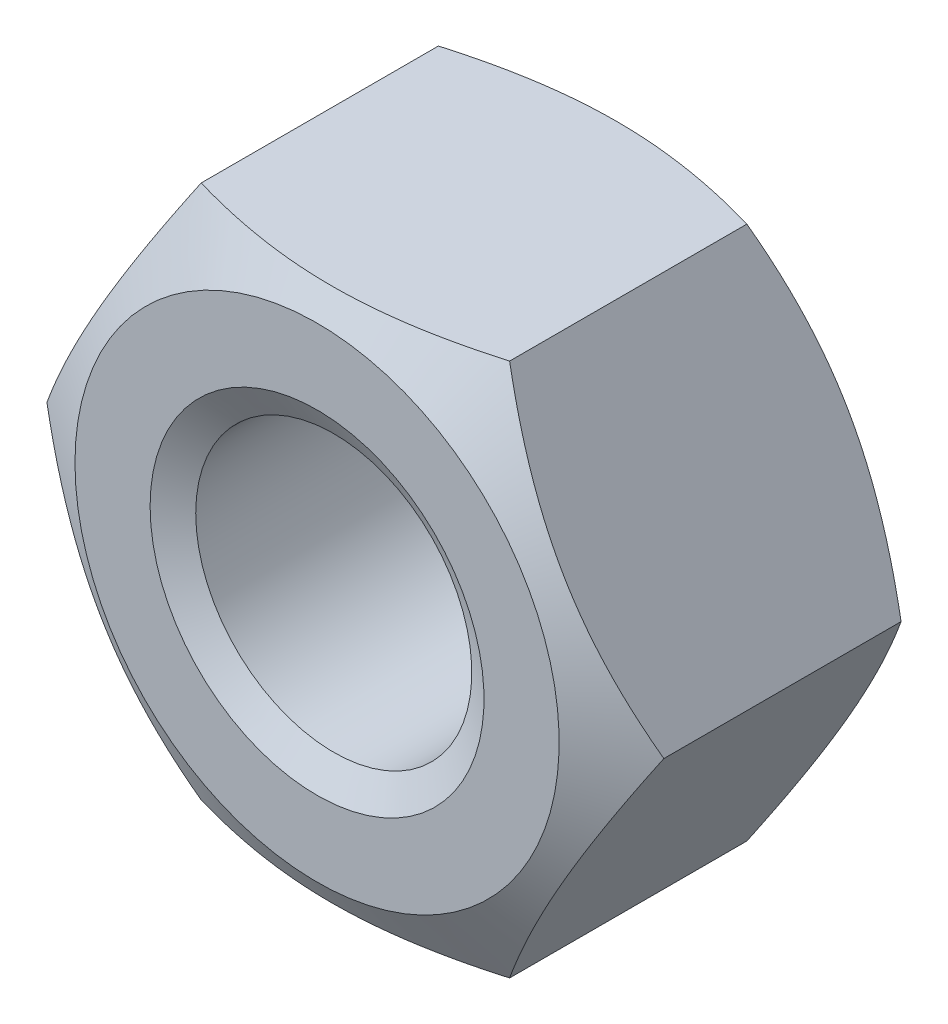
SolidWorks part; units mm, degrees
ref_plane "Front" through (0, 0, 0) normal (0, 0, 1) x (1, 0, 0)
ref_plane "Top" through (0, 0, 0) normal (0, 1, 0) x (1, 0, 0)
ref_plane "Right" through (0, 0, 0) normal (1, 0, 0) x (0, 0, -1)
sketch "Sketch1" plane through (0, 0, 0) normal (0, 0, 1) x (1, 0, 0)
  line L1 (4.6188, 0) -> (2.3094, 4)
  line L2 (2.3094, 4) -> (-2.3094, 4)
  line L3 (-2.3094, 4) -> (-4.6188, 0)
  line L4 (-4.6188, 0) -> (-2.3094, -4)
  line L5 (-2.3094, -4) -> (2.3094, -4)
  line L6 (2.3094, -4) -> (4.6188, 0)
  circle A0 centre (0, 0) radius 4 construction
  circle A1 centre (0, 0) radius 2.067
extrude "BaseNut" add sketch "Sketch1" against normal blind 4.7
cosmetic thread "ThreadCosmetic1" [suppressed] parameters "D"=5
sketch "Sketch2" plane through (0, 0, 0) normal (0, 1, 0) x (1, 0, 0)
  line L0 (-4.6188, 4.7) -> (-3.625, 4.7)
  line L2 (-3.625, 4.7) -> (-4.6188, 4.1262)
  line L3 (-4.6188, 4.1262) -> (-4.6188, 4.7)
  line L4 (0, 3.3759) -> (0, -9.8171) construction
  line L6 (-9.7712, 2.35) -> (9.8853, 2.35) construction
  line L7 (-4.6188, 0.5738) -> (-4.6188, 0)
  line L8 (-3.625, 0) -> (-4.6188, 0.5738)
  line L9 (-4.6188, 0) -> (-3.625, 0)
revolve "Double-Chamfer" cut sketch "Sketch2" angle 360 about L4
chamfer "EndChamfer" distance 0.433 angle 30 2 edges at (2.067, 0, -4.7) (2.067, 0, 0)
sketch "Sketch3" plane through (0, 0, 0) normal (0, 1, 0) x (1, 0, 0)
  line L0 (-2.442, 4.267) -> (-2.067, 4.0505)
  line L1 (-2.067, 4.0505) -> (-1.634, 4.0505)
  line L2 (-1.634, 4.0505) -> (-1.634, 4.4835)
  line L3 (-1.634, 4.4835) -> (-2.067, 4.4835)
  line L4 (-2.067, 4.4835) -> (-2.442, 4.267)
  line L5 (0, 7.4383) -> (0, 16.8806) construction
revolve "Cut-Revolve10" [suppressed] cut sketch "Sketch3" angle 360 about L5
pattern_linear "LPattern10" [suppressed] count 9 spacing 0.5196 along (0, 0, -1)
equation "\"dw@Sketch2\" = \"s@Sketch1\"-0.75"
equation "\"D2@Sketch2\" = \"m@BaseNut\" / 2"
equation "\"D2@Sketch3\" = \"D@Sketch1\""
equation "\"D1@Sketch3\" =  (\"D@ThreadCosmetic1\"   - \"D@Sketch1\")  / 2"
equation "\"D3@LPattern10\" = \"D1@Sketch3\" * 1.2"
equation "\"D1@LPattern10\" = \"m@BaseNut\"/\"D3@LPattern10\""
